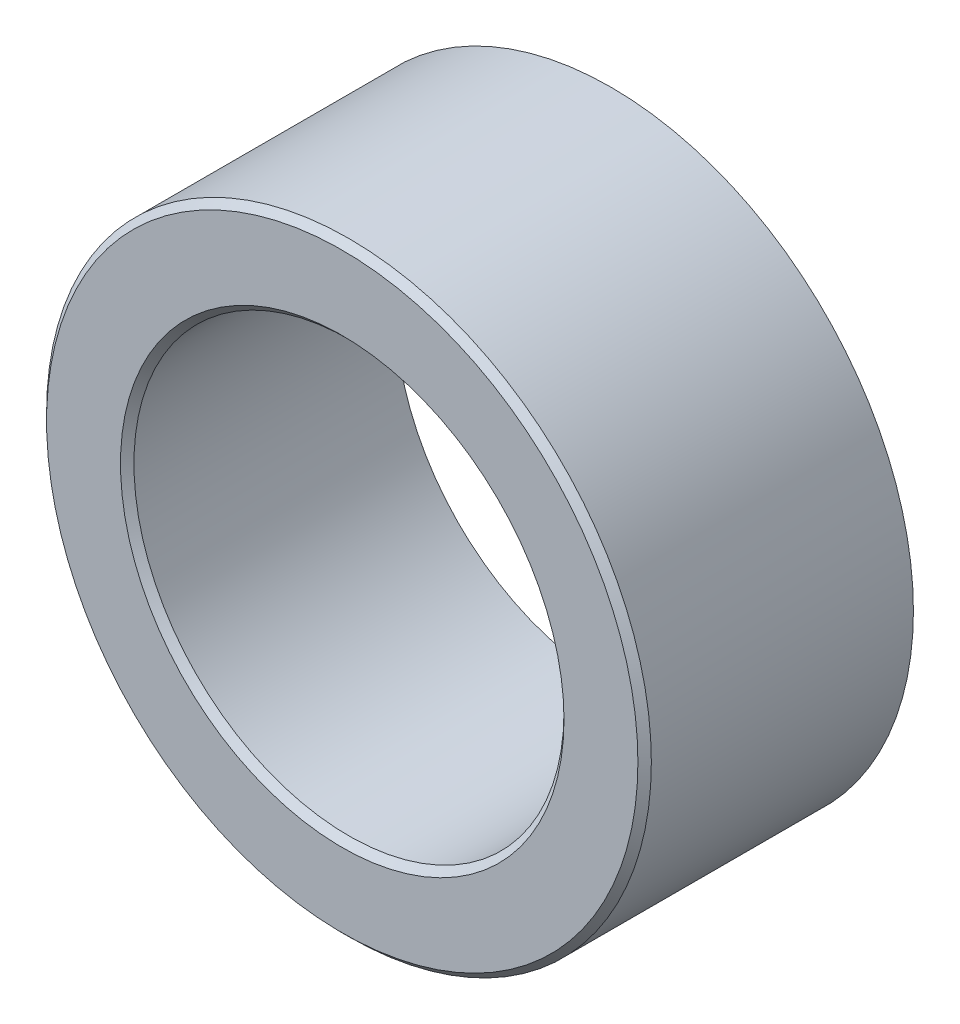
SolidWorks part; units mm, degrees
material "1023 碳钢板 (SS)"
ref_plane "前视基准面" through (0, 0, 0) normal (0, 0, 1) x (1, 0, 0)
ref_plane "上视基准面" through (0, 0, 0) normal (0, 1, 0) x (1, 0, 0)
ref_plane "右视基准面" through (0, 0, 0) normal (1, 0, 0) x (0, 0, -1)
sketch "草图1" plane through (0, 0, 0) normal (0, 0, 1) x (1, 0, 0)
  circle A0 centre (0, 0) radius 22.5
  dimension "D1" = 45
extrude "凸台-拉伸1" add sketch "草图1" along normal blind 20
sketch "草图2" plane through (0, 0, 20) normal (0, 0, 1) x (1, 0, 0)
  circle A0 centre (0, 0) radius 16
  dimension "D1" = 32
extrude "切除-拉伸1" cut sketch "草图2" against normal blind 20
chamfer "倒角1" distance 0.5 angle 45 1 edges at (16, 0, 20)
chamfer "倒角2" distance 0.5 angle 45 1 edges at (22.5, 0, 20)
